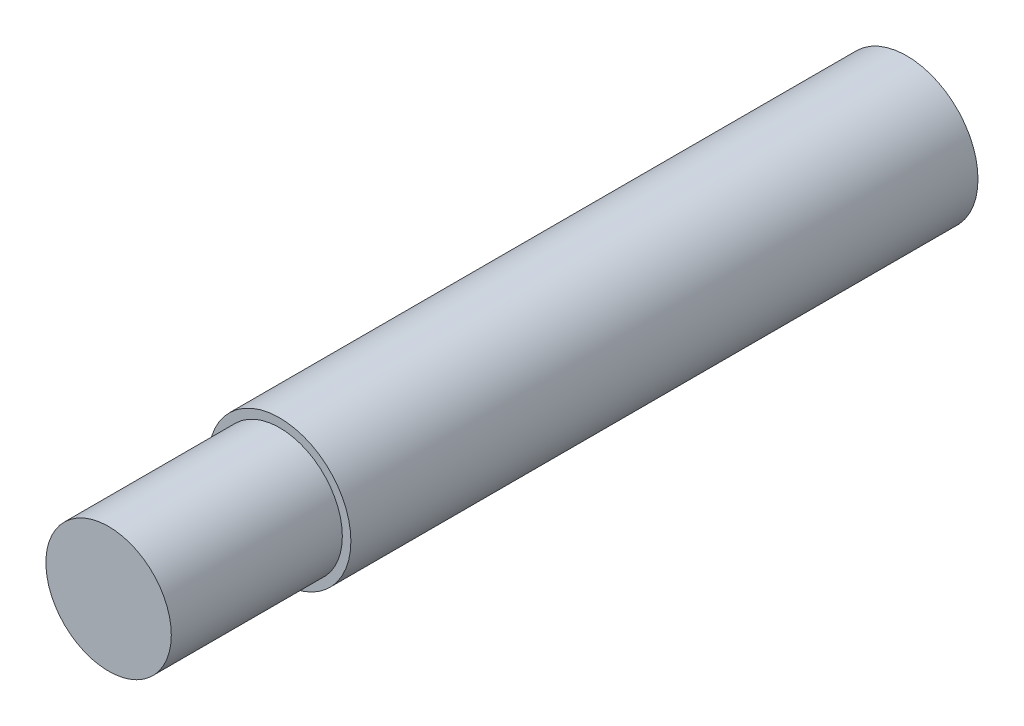
SolidWorks part; units mm, degrees
material "1060 合金"
ref_plane "前视基准面" through (0, 0, 0) normal (0, 0, 1) x (1, 0, 0)
ref_plane "上视基准面" through (0, 0, 0) normal (0, 1, 0) x (1, 0, 0)
ref_plane "右视基准面" through (0, 0, 0) normal (1, 0, 0) x (0, 0, -1)
sketch "草图1" plane through (0, 0, 0) normal (0, 0, 1) x (1, 0, 0)
  circle A0 centre (0, 0) radius 1.25
extrude "凸台-拉伸1" add sketch "草图1" along normal blind 11
sketch "草图2" plane through (0, 0, 11) normal (0, 0, 1) x (1, 0, 0)
  circle A0 centre (0, 0) radius 1.1
extrude "凸台-拉伸2" add sketch "草图2" along normal blind 3
